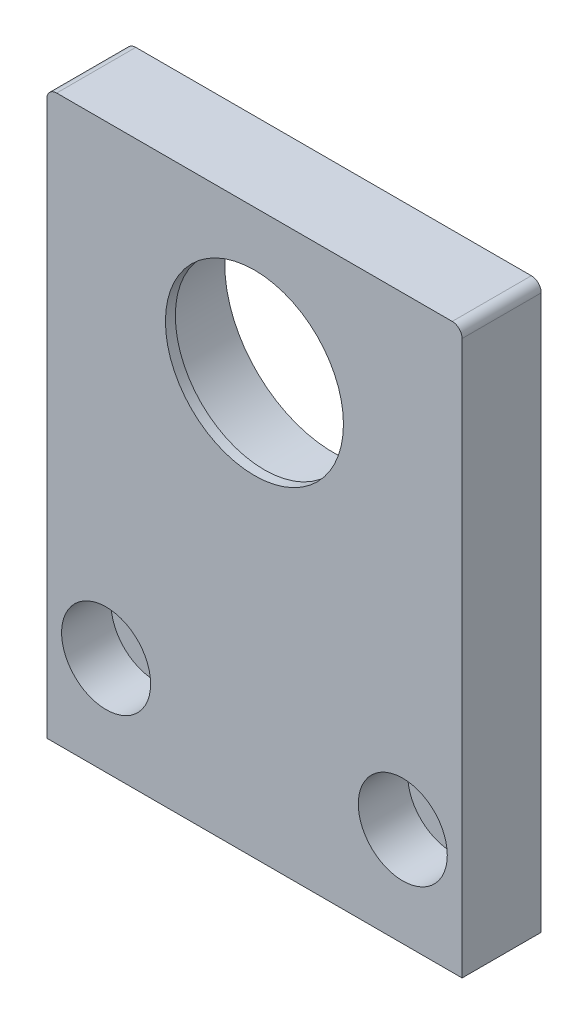
SolidWorks part; units mm, degrees
ref_plane "Front Plane" through (0, 0, 0) normal (0, 0, 1) x (1, 0, 0)
ref_plane "Top Plane" through (0, 0, 0) normal (0, 1, 0) x (1, 0, 0)
ref_plane "Right Plane" through (0, 0, 0) normal (1, 0, 0) x (0, 0, -1)
sketch "Sketch1" plane through (0, 0, 0) normal (0, 0, 1) x (1, 0, 0)
  line L0 (0, 28.5) -> (0, -28.5) construction
  line L1 (-20, 28.5) -> (20, 28.5)
  line L2 (-21, 27.5) -> (-21, -28.5)
  line L3 (-21, -28.5) -> (21, -28.5)
  line L4 (21, 27.5) -> (21, -28.5)
  line L5 (-21, 28.5) -> (21, -28.5) construction
  line L6 (-21, -28.5) -> (21, 28.5) construction
  line L7 (-31.1244, -18.5) -> (49.6543, -18.5) construction
  circle A0 centre (0, 14) radius 9
  circle A1 centre (-15, -18.5) radius 2.5
  circle A2 centre (15, -18.5) radius 2.5
  arc A3 (20, 28.5) -> (21, 27.5) centre (20, 27.5) cw
  arc A4 (-20, 28.5) -> (-21, 27.5) centre (-20, 27.5) ccw
  point P0 (0, 0)
  dimension "D3" = 18
  dimension "D5" = 5
  dimension "D6" = 5
  dimension "D10" = 1
  dimension "D1" = 42
  dimension "D2" = 57
  dimension "D4" = 10
  dimension "D7" = 6
  dimension "D8" = 6
  dimension "D9" = 42.5
extrude "Boss-Extrude1" add sketch "Sketch1" along normal blind 8
sketch "Sketch2" plane through (0, 0, 8) normal (0, 0, 1) x (1, 0, 0)
  circle A0 centre (-15, -18.5) radius 4.5
  circle A1 centre (15, -18.5) radius 4.5
  dimension "D1" = 9
  dimension "D2" = 9
extrude "Cut-Extrude1" cut sketch "Sketch2" against normal blind 5
sketch "Sketch3" plane through (0, 0, 0) normal (0, 0, -1) x (-1, 0, 0)
  circle A0 centre (0, 14) radius 11
  dimension "D1" = 22
extrude "Cut-Extrude2" cut sketch "Sketch3" against normal blind 7
